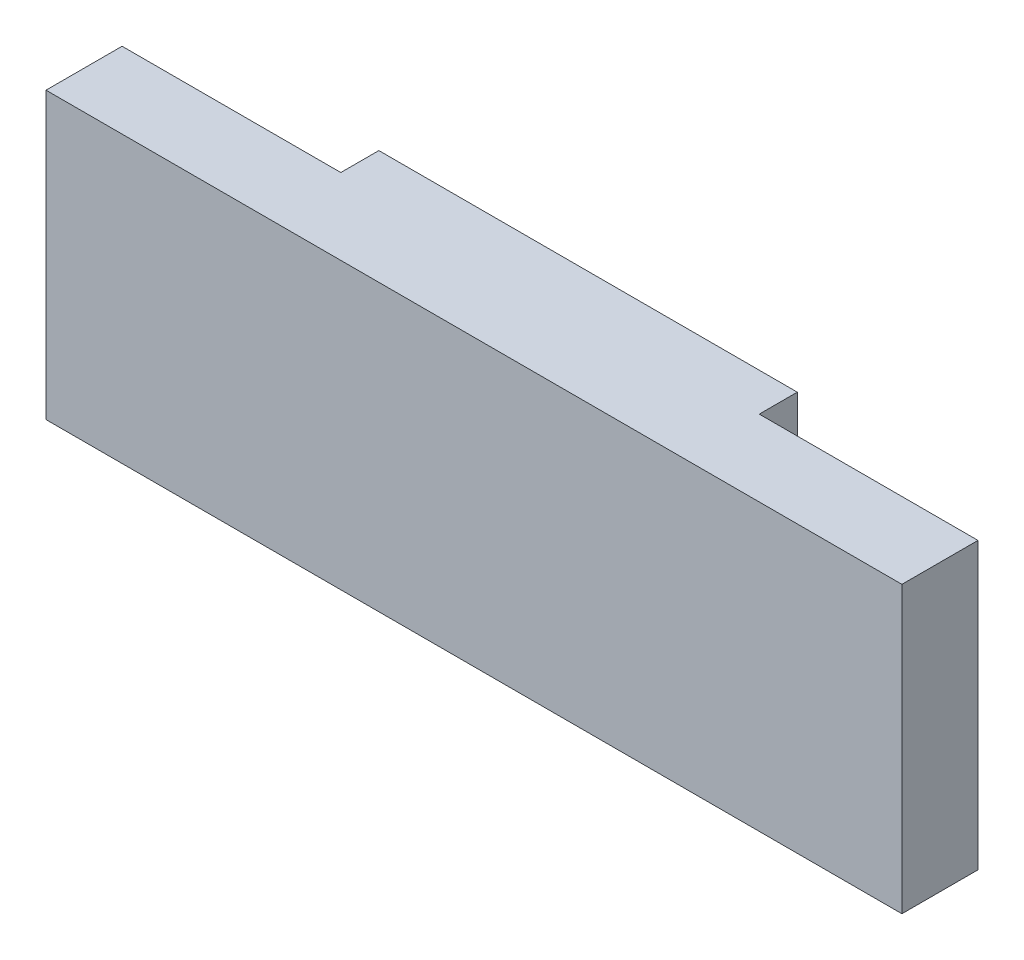
from build123d import *

# Parameters (mm, degrees)
BOSS_EXTRUDE1_DEPTH = 150


with BuildPart() as part:
    # Sketch1 → Boss-Extrude1 (new body)
    with BuildSketch(Plane(origin=(0, 0, 0), x_dir=(1, 0, 0), z_dir=(0, 1, 0))):
        Polygon((115, 0), (115, 20), (335, 20), (335, 0), (450, 0), (450, -40), (0, -40), (0, 0), align=None)
    extrude(amount=BOSS_EXTRUDE1_DEPTH)


solid = part.part
